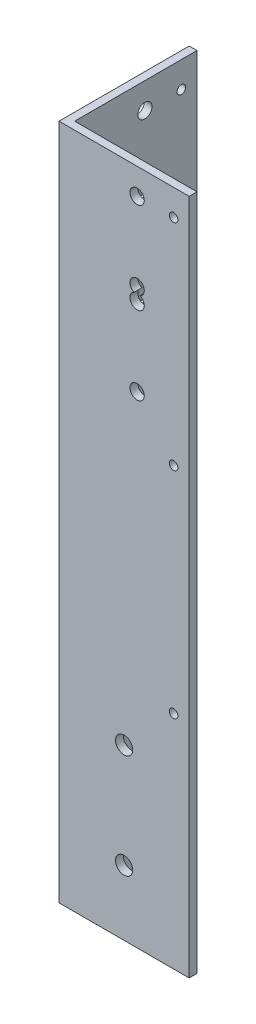
from build123d import *

# Parameters (mm, degrees)
EXTRUDE_1_DEPTH    = 260
HOLE_WIZARD_M5_1_D = 5.5
HOLE_WIZARD_M5_2_D = 5.5
HOLE_WIZARD_M6_1_D = 6.6
HOLE_WIZARD_M6_2_D = 6.6
HOLE_WIZARD_M4_1_D = 3.3
HOLE_WIZARD_M4_2_D = 3.3


with BuildPart() as part:
    # 草图1 → 凸台-拉伸1 (new body)
    with BuildSketch(Plane(origin=(0, 0, 0), x_dir=(1, 0, 0), z_dir=(0, 1, 0))):
        Polygon((0, 0), (50, 0), (50, 3), (3, 3), (3, 50), (0, 50), align=None)
    extrude(amount=EXTRUDE_1_DEPTH)

    # M5 间隙孔1 (through all)
    with Locations(Plane(origin=(0, 0, -3), x_dir=(-1, 0, 0), z_dir=(0, 0, -1))):
        with Locations((-30, 250), (-30, 215), (-30, 220), (-30, 185)):
            Hole(HOLE_WIZARD_M5_1_D / 2)

    # M5 间隙孔2 (through all)
    with Locations(Plane(origin=(3, 0, 0), x_dir=(0, 0, -1), z_dir=(1, 0, 0))):
        with Locations((30, 220), (30, 185), (30, 250), (30, 215)):
            Hole(HOLE_WIZARD_M5_2_D / 2)

    # M6 间隙孔1 (through all)
    with Locations(Plane.XY):
        with Locations((25, 65), (25, 25)):
            Hole(HOLE_WIZARD_M6_1_D / 2)

    # M6 间隙孔2 (through all)
    with Locations(Plane.ZY):
        with Locations((-25, 65), (-25, 25)):
            Hole(HOLE_WIZARD_M6_2_D / 2)

    # M4 螺纹孔1 (through all)
    with Locations(Plane(origin=(0, 0, -3), x_dir=(-1, 0, 0), z_dir=(0, 0, -1))):
        with Locations((-44, 250), (-44, 167.5), (-44, 85)):
            Hole(HOLE_WIZARD_M4_1_D / 2)

    # M4 螺纹孔2 (through all)
    with Locations(Plane(origin=(3, 0, 0), x_dir=(0, 0, -1), z_dir=(1, 0, 0))):
        with Locations((44, 250), (44, 167.5), (44, 85)):
            Hole(HOLE_WIZARD_M4_2_D / 2)


solid = part.part
